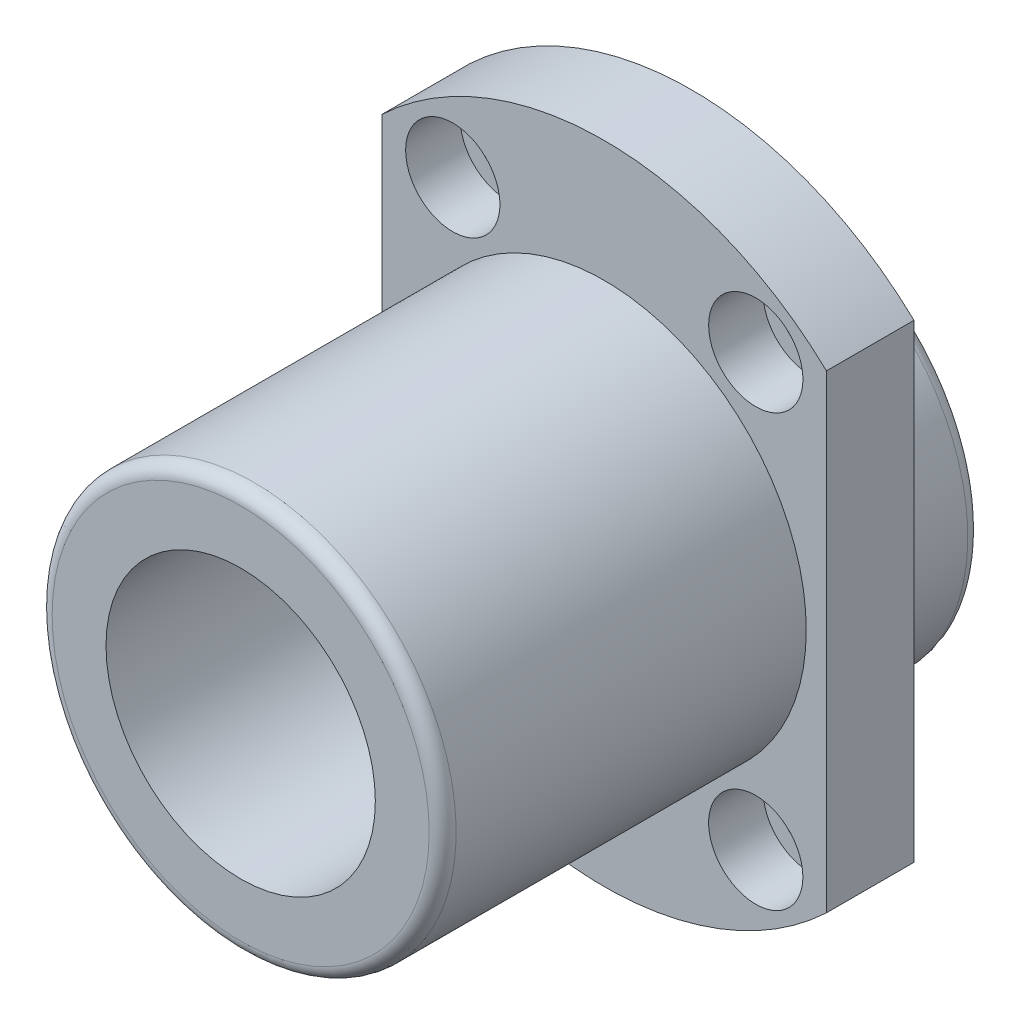
from build123d import *

# Parameters (mm, degrees)
EXTRUDE_START   = 13
SKETCH_2_R      = 30
EXTRUDE_1_DEPTH = 13


with BuildPart() as part:
    # 草图1 → 旋转1 (revolve)
    with BuildSketch(Plane(origin=(0, 0, 0), x_dir=(0, 0, -1), z_dir=(1, 0, 0)), mode=Mode.PRIVATE) as revolve_1_sk:
        with BuildLine():
            Line((-67, 28), (-67, 20))
            Line((-67, 20), (13, 20))
            Line((13, 20), (13, 28))
            ThreePointArc((13, 28), (12.414213562, 29.414213562), (11, 30))
            Line((11, 30), (-65, 30))
            ThreePointArc((-65, 30), (-66.414213562, 29.414213562), (-67, 28))
        make_face()
    revolve(revolve_1_sk.sketch.rotate(Axis((0, 0, -13), (0, 0, 1)), 90), axis=Axis((0, 0, -13), (0, 0, 1)))

    # 草图2 → 凸台-拉伸1 (add)
    with BuildSketch(Plane.XY.offset(EXTRUDE_START)):
        with BuildLine():
            Line((-33, 34.856850116), (-33, -34.856850116))
            ThreePointArc((-33, -34.856850116), (0, -48), (33, -34.856850116))
            Line((33, -34.856850116), (33, 34.856850116))
            ThreePointArc((33, 34.856850116), (0, 48), (-33, 34.856850116))
        make_face()
        with Locations(Location((0, 0, 0), (0, 0, 180))):
            Circle(SKETCH_2_R, mode=Mode.SUBTRACT)
    extrude(amount=-EXTRUDE_1_DEPTH)

    # 草图3 → 切除-旋转1 (revolve, cut)
    with BuildSketch(Plane(origin=(-22.5, 0, 0), x_dir=(0, 0, -1), z_dir=(1, 0, 0)), mode=Mode.PRIVATE) as cut_revolve_1_sk:
        Polygon((-13, 32), (-13, 39), (-4.9, 39), (-4.9, 36.5), (0, 36.5), (0, 32), align=None)
    revolve(cut_revolve_1_sk.sketch.rotate(Axis((-22.5, 32, 0), (0, 0, 1)), 90), axis=Axis((-22.5, 32, 0), (0, 0, 1)), mode=Mode.SUBTRACT)

    # 草图4 → 切除-旋转2 (revolve, cut)
    with BuildSketch(Plane(origin=(-22.5, 0, 0), x_dir=(0, 0, -1), z_dir=(1, 0, 0)), mode=Mode.PRIVATE) as cut_revolve_2_sk:
        Polygon((0, -32), (0, -36.5), (-4.9, -36.5), (-4.9, -39), (-13, -39), (-13, -32), align=None)
    revolve(cut_revolve_2_sk.sketch.rotate(Axis((-22.5, -32, 13), (0, 0, -1)), 270), axis=Axis((-22.5, -32, 13), (0, 0, -1)), mode=Mode.SUBTRACT)

    # 草图5 → 切除-旋转3 (revolve, cut)
    with BuildSketch(Plane(origin=(22.5, 0, 0), x_dir=(0, 0, -1), z_dir=(1, 0, 0)), mode=Mode.PRIVATE) as cut_revolve_3_sk:
        Polygon((-13, 32), (-13, 39), (-4.9, 39), (-4.9, 36.5), (0, 36.5), (0, 32), align=None)
    revolve(cut_revolve_3_sk.sketch.rotate(Axis((22.5, 32, 0), (0, 0, 1)), 90), axis=Axis((22.5, 32, 0), (0, 0, 1)), mode=Mode.SUBTRACT)

    # 草图6 → 切除-旋转4 (revolve, cut)
    with BuildSketch(Plane(origin=(22.5, 0, 0), x_dir=(0, 0, -1), z_dir=(1, 0, 0)), mode=Mode.PRIVATE) as cut_revolve_4_sk:
        Polygon((0, -32), (0, -36.5), (-4.9, -36.5), (-4.9, -39), (-13, -39), (-13, -32), align=None)
    revolve(cut_revolve_4_sk.sketch.rotate(Axis((22.5, -32, 13), (0, 0, -1)), 270), axis=Axis((22.5, -32, 13), (0, 0, -1)), mode=Mode.SUBTRACT)


solid = part.part
